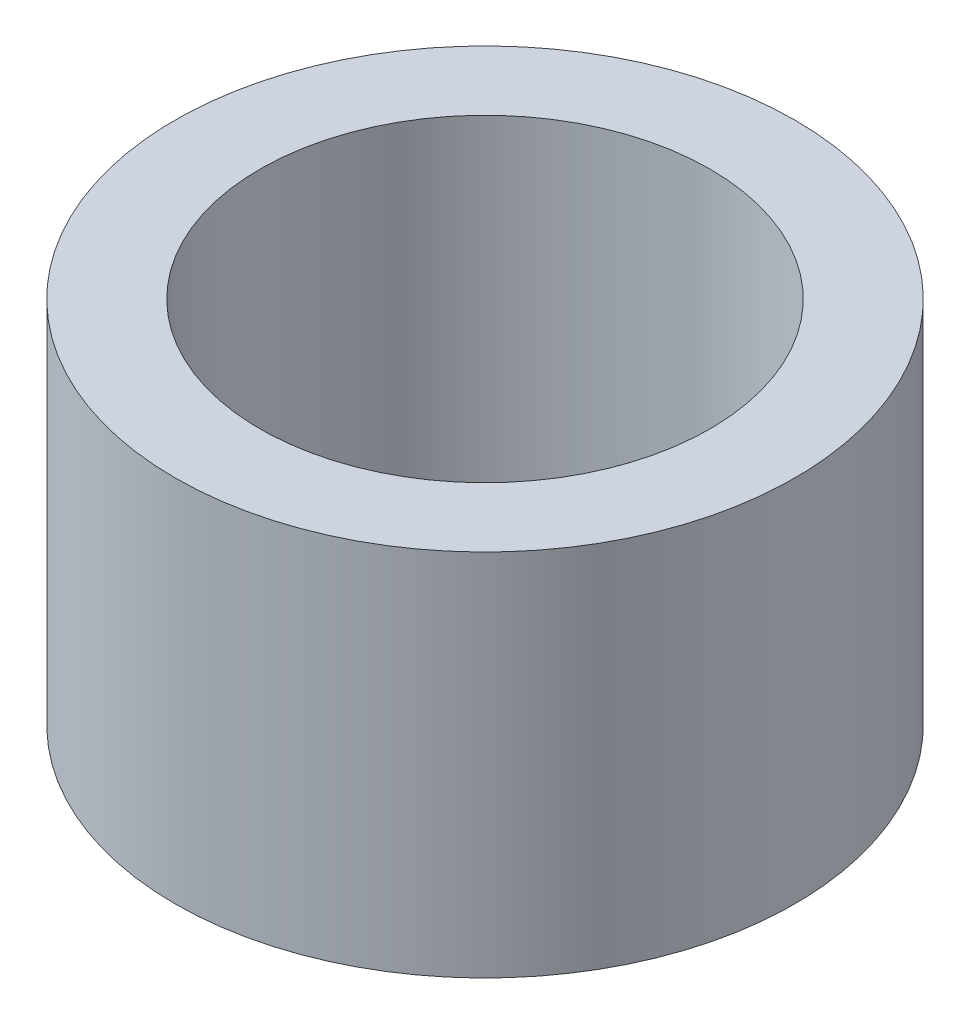
from build123d import *

# Parameters (mm, degrees)
SKETCH1_W = 1.15
SKETCH1_H = 5


with BuildPart() as part:
    # Sketch1 → Revolve1 (revolve)
    with BuildSketch(Plane.XY, mode=Mode.PRIVATE) as revolve1_sk:
        with Locations((3.625, 0)):
            Rectangle(SKETCH1_W, SKETCH1_H)
    revolve(revolve1_sk.sketch.rotate(Axis((0, 0, 0), (0, 1, 0)), 90), axis=Axis((0, 0, 0), (0, 1, 0)))


solid = part.part
